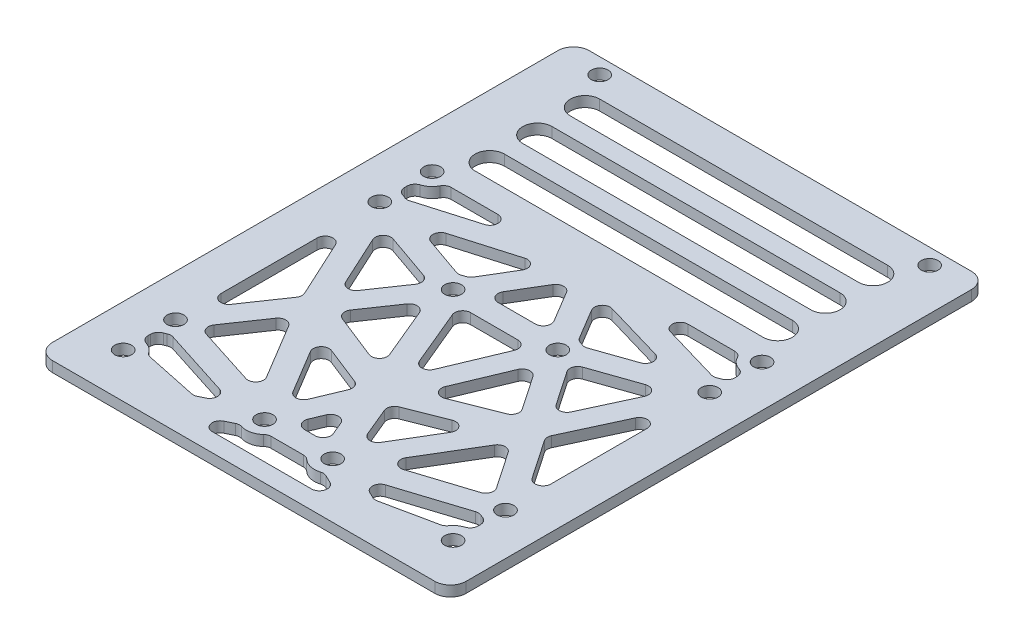
SolidWorks part; units mm, degrees
material "Thornel Mat VMA"
ref_plane "Front Plane" through (0, 0, 0) normal (0, 0, 1) x (1, 0, 0)
ref_plane "Top Plane" through (0, 0, 0) normal (0, 1, 0) x (1, 0, 0)
ref_plane "Right Plane" through (0, 0, 0) normal (1, 0, 0) x (0, 0, -1)
sketch "Sketch1" plane through (0, 0, 0) normal (0, 1, 0) x (1, 0, 0)
  line L0 (0, 56) -> (0, -46.5) construction
  line L1 (-39.5, 56) -> (39.5, 56)
  line L2 (-39.5, 56) -> (-39.5, -46.5)
  line L3 (-39.5, -46.5) -> (39.5, -46.5)
  line L4 (39.5, 56) -> (39.5, -46.5)
  line L5 (-31.5, 21) -> (-31.5, 11) construction
  line L6 (31.5, 21) -> (31.5, 11) construction
  line L7 (-10, 3.5) -> (10, 3.5) construction
  line L8 (-6.5, -36) -> (6.5, -36) construction
  line L9 (-31.5, -28) -> (-31.5, -38) construction
  line L10 (31.5, -28) -> (31.5, -38) construction
  circle A0 centre (-31.5, 11) radius 1.6
  circle A1 centre (-31.5, 21) radius 1.6
  circle A2 centre (31.5, 11) radius 1.6
  circle A3 centre (31.5, 21) radius 1.6
  circle A4 centre (-6.5, -36) radius 1.6
  circle A5 centre (6.5, -36) radius 1.6
  circle A6 centre (-10, 3.5) radius 1.6
  circle A7 centre (10, 3.5) radius 1.6
  circle A8 centre (-31.5, 53) radius 1.6
  circle A9 centre (31.5, 53) radius 1.6
  circle A10 centre (-31.5, -28) radius 1.6
  circle A11 centre (-31.5, -38) radius 1.6
  circle A12 centre (31.5, -38) radius 1.6
  circle A13 centre (31.5, -28) radius 1.6
  dimension "D2" = 8
  dimension "D3" = 3.2
  dimension "D5" = 20
  dimension "D12" = 3
  dimension "D13" = 2
  dimension "D1" = 79
  dimension "D4" = 10
  dimension "D6" = 3.5
  dimension "D7" = 52.5
  dimension "D8" = 46.5
  dimension "D9" = 13
  dimension "D10" = 10.5
  dimension "D11" = 11
  dimension "D14" = 28
extrude "Boss-Extrude1" add sketch "Sketch1" along normal blind 2
sketch "Sketch2" plane through (0, 2, 0) normal (0, 1, 0) x (1, 0, 0)
  line L0 (0, 56) -> (0, -46.5) construction
  line L1 (39.5, 56) -> (-39.5, 56) construction
  line L2 (-39.5, -46.5) -> (39.5, -46.5) construction
  line L3 (-27.5, 46.2) -> (27.5, 46.2) construction
  line L4 (-27.5, 49) -> (27.5, 49)
  line L5 (-27.5, 43.4) -> (27.5, 43.4)
  line L6 (-39.5, 56) -> (-39.5, -46.5) construction
  line L7 (-27.5, 37.1) -> (27.5, 37.1) construction
  line L8 (-27.5, 39.9) -> (27.5, 39.9)
  line L9 (-27.5, 34.3) -> (27.5, 34.3)
  line L10 (-27.5, 28) -> (27.5, 28) construction
  line L11 (-27.5, 30.8) -> (27.5, 30.8)
  line L12 (-27.5, 25.2) -> (27.5, 25.2)
  line L13 (-31.5, -38) -> (-16.9387, -41.0657) construction
  line L16 (-16, -43) -> (16, -43)
  line L19 (-31.0571, -35.8961) -> (-16.4957, -38.9619)
  line L22 (-31.9429, -40.1039) -> (-17.3816, -43.1696)
  line L25 (-31.5, 11) -> (-10, 3.5) construction
  line L28 (-30.7918, 13.03) -> (-9.2918, 5.53)
  line L31 (-10, 3.5) -> (10, 3.5) construction
  line L32 (-10, 5.65) -> (10, 5.65)
  line L33 (-10, 1.35) -> (10, 1.35)
  line L37 (-32.2082, 8.97) -> (-10.7082, 1.47)
  line L43 (-16.9387, -41.0657) -> (-6.5, -36) construction
  line L44 (-17.8773, -39.1315) -> (-7.4387, -34.0657)
  line L45 (-16, -43) -> (-5.5613, -37.9343)
  line L46 (16.9387, -41.0657) -> (6.5, -36) construction
  line L49 (-31.5, -28) -> (-10, 3.5) construction
  line L56 (-33.2758, -26.788) -> (-11.7758, 4.712)
  line L59 (-29.7242, -29.212) -> (-8.2242, 2.288)
  line L62 (-31.5, 11) -> (-31.5, -28)
  line L65 (-31.5, -28) -> (-6.5, -36) construction
  line L68 (-6.5, -36) -> (6.5, -36) construction
  line L69 (-6.5, -33.85) -> (6.5, -33.85)
  line L70 (-6.5, -38.15) -> (6.5, -38.15)
  line L71 (-30.8447, -25.9523) -> (-5.8447, -33.9523)
  line L72 (-32.1553, -30.0477) -> (-7.1553, -38.0477)
  line L73 (-31.5, -28) -> (-31.5, -38)
  line L74 (17.8773, -39.1315) -> (7.4387, -34.0657)
  line L75 (16, -43) -> (5.5613, -37.9343)
  line L76 (-10, 3.5) -> (6.5, -36) construction
  line L77 (-8.0161, 4.3287) -> (8.4839, -35.1713)
  line L78 (-11.9839, 2.6713) -> (4.5161, -36.8287)
  line L79 (-6.5, -36) -> (10, 3.5) construction
  line L80 (-8.4839, -35.1713) -> (8.0161, 4.3287)
  line L81 (-4.5161, -36.8287) -> (11.9839, 2.6713)
  line L82 (-31.5, 11) -> (-20.75, -12.25) construction
  line L83 (-29.5485, 11.9023) -> (-18.7985, -11.3477)
  line L84 (-33.4515, 10.0977) -> (-22.7015, -13.1523)
  line L85 (-20.75, -12.25) -> (-6.5, -36) construction
  line L86 (-18.9064, -11.1438) -> (-4.6564, -34.8938)
  line L87 (-22.5936, -13.3562) -> (-8.3436, -37.1062)
  line L88 (-20.75, -12.25) -> (0, -20.4394) construction
  line L89 (-19.9607, -10.2501) -> (0.7893, -18.4395)
  line L90 (-21.5393, -14.2499) -> (-0.7893, -22.4393)
  line L91 (-28.0927, 20.2) -> (28.0927, 20.2)
  line L92 (-31.5, 17.5) -> (-31.5, 14.5)
  line L93 (31.5, 17.5) -> (31.5, 14.5)
  line L94 (-31.5, 11) -> (0, 20.2) construction
  line L95 (-32.1028, 13.0638) -> (-0.6028, 22.2638)
  line L96 (-30.8972, 8.9362) -> (0.6028, 18.1362)
  line L97 (-10, 3.5) -> (0, 20.2) construction
  line L98 (-11.8446, 4.6045) -> (-1.8446, 21.3045)
  line L99 (-8.1554, 2.3955) -> (1.8446, 19.0955)
  line L100 (31.5, -28) -> (31.5, -38)
  line L101 (31.5, 11) -> (31.5, -28)
  line L102 (31.5, -38) -> (16.9387, -41.0657) construction
  line L103 (31.0571, -35.8961) -> (16.4957, -38.9619)
  line L104 (31.9429, -40.1039) -> (17.3816, -43.1696)
  line L105 (31.5, -28) -> (6.5, -36) construction
  line L106 (30.8447, -25.9523) -> (5.8447, -33.9523)
  line L107 (32.1553, -30.0477) -> (7.1553, -38.0477)
  line L108 (20.75, -12.25) -> (0, -20.4394) construction
  line L109 (19.9607, -10.2501) -> (-0.7893, -18.4395)
  line L110 (21.5393, -14.2499) -> (0.7893, -22.4393)
  line L111 (20.75, -12.25) -> (6.5, -36) construction
  line L112 (18.9064, -11.1438) -> (4.6564, -34.8938)
  line L113 (22.5936, -13.3562) -> (8.3436, -37.1062)
  line L114 (31.5, -28) -> (10, 3.5) construction
  line L115 (33.2758, -26.788) -> (11.7758, 4.712)
  line L116 (29.7242, -29.212) -> (8.2242, 2.288)
  line L117 (31.5, 11) -> (20.75, -12.25) construction
  line L118 (29.5485, 11.9023) -> (18.7985, -11.3477)
  line L119 (33.4515, 10.0977) -> (22.7015, -13.1523)
  line L120 (31.5, 11) -> (10, 3.5) construction
  line L121 (30.7918, 13.03) -> (9.2918, 5.53)
  line L122 (32.2082, 8.97) -> (10.7082, 1.47)
  line L123 (10, 3.5) -> (0, 20.2) construction
  line L124 (11.8446, 4.6045) -> (1.8446, 21.3045)
  line L125 (8.1554, 2.3955) -> (-1.8446, 19.0955)
  line L126 (31.5, 11) -> (0, 20.2) construction
  line L127 (32.1028, 13.0638) -> (0.6028, 22.2638)
  line L128 (30.8972, 8.9362) -> (-0.6028, 18.1362)
  arc A0 (-27.5, 49) -> (-27.5, 43.4) centre (-27.5, 46.2) ccw
  arc A1 (27.5, 43.4) -> (27.5, 49) centre (27.5, 46.2) ccw
  arc A2 (-27.5, 39.9) -> (-27.5, 34.3) centre (-27.5, 37.1) ccw
  arc A3 (27.5, 34.3) -> (27.5, 39.9) centre (27.5, 37.1) ccw
  arc A4 (-27.5, 30.8) -> (-27.5, 25.2) centre (-27.5, 28) ccw
  arc A5 (27.5, 25.2) -> (27.5, 30.8) centre (27.5, 28) ccw
  arc A18 (-10, 5.65) -> (-10, 1.35) centre (-10, 3.5) ccw
  arc A19 (10, 1.35) -> (10, 5.65) centre (10, 3.5) ccw
  arc A26 (-17.8773, -39.1315) -> (-16, -43) centre (-16.9387, -41.0657) ccw
  arc A27 (-5.5613, -37.9343) -> (-7.4387, -34.0657) centre (-6.5, -36) ccw
  circle A44 centre (-10, 3.5) radius 3.5
  circle A45 centre (-31.5, 11) radius 3.5
  circle A46 centre (-6.5, -36) radius 3.5
  circle A48 centre (10, 3.5) radius 3.5
  circle A49 centre (31.5, 11) radius 3.5
  circle A50 centre (6.5, -36) radius 3.5
  arc A54 (-6.5, -33.85) -> (-6.5, -38.15) centre (-6.5, -36) ccw
  arc A55 (6.5, -38.15) -> (6.5, -33.85) centre (6.5, -36) ccw
  circle A56 centre (-31.5, -28) radius 3.5
  circle A57 centre (-31.5, -38) radius 3.5
  circle A58 centre (31.5, -28) radius 3.5
  circle A59 centre (31.5, -38) radius 3.5
  arc A60 (-31.0571, -35.8961) -> (-31.9429, -40.1039) centre (-31.5, -38) ccw
  arc A61 (-17.3816, -43.1696) -> (-16.4957, -38.9619) centre (-16.9387, -41.0657) ccw
  arc A62 (-30.7918, 13.03) -> (-32.2082, 8.97) centre (-31.5, 11) ccw
  arc A63 (-10.7082, 1.47) -> (-9.2918, 5.53) centre (-10, 3.5) ccw
  arc A64 (-33.2758, -26.788) -> (-29.7242, -29.212) centre (-31.5, -28) ccw
  arc A65 (-8.2242, 2.288) -> (-11.7758, 4.712) centre (-10, 3.5) ccw
  arc A66 (-30.8447, -25.9523) -> (-32.1553, -30.0477) centre (-31.5, -28) ccw
  arc A67 (-7.1553, -38.0477) -> (-5.8447, -33.9523) centre (-6.5, -36) ccw
  arc A68 (17.8773, -39.1315) -> (16, -43) centre (16.9387, -41.0657) cw
  arc A69 (5.5613, -37.9343) -> (7.4387, -34.0657) centre (6.5, -36) cw
  arc A70 (-8.0161, 4.3287) -> (-11.9839, 2.6713) centre (-10, 3.5) ccw
  arc A71 (4.5161, -36.8287) -> (8.4839, -35.1713) centre (6.5, -36) ccw
  arc A72 (-8.4839, -35.1713) -> (-4.5161, -36.8287) centre (-6.5, -36) ccw
  arc A73 (11.9839, 2.6713) -> (8.0161, 4.3287) centre (10, 3.5) ccw
  arc A74 (-29.5485, 11.9023) -> (-33.4515, 10.0977) centre (-31.5, 11) ccw
  arc A75 (-22.7015, -13.1523) -> (-18.7985, -11.3477) centre (-20.75, -12.25) ccw
  arc A76 (-18.9064, -11.1438) -> (-22.5936, -13.3562) centre (-20.75, -12.25) ccw
  arc A77 (-8.3436, -37.1062) -> (-4.6564, -34.8938) centre (-6.5, -36) ccw
  arc A78 (-19.9607, -10.2501) -> (-21.5393, -14.2499) centre (-20.75, -12.25) ccw
  arc A79 (-0.7893, -22.4393) -> (0.7893, -18.4395) centre (0, -20.4394) ccw
  circle A80 centre (-31.5, 21) radius 3.5
  circle A81 centre (31.5, 21) radius 3.5
  arc A82 (-32.1028, 13.0638) -> (-30.8972, 8.9362) centre (-31.5, 11) ccw
  arc A83 (0.6028, 18.1362) -> (-0.6028, 22.2638) centre (0, 20.2) ccw
  arc A84 (-11.8446, 4.6045) -> (-8.1554, 2.3955) centre (-10, 3.5) ccw
  arc A85 (1.8446, 19.0955) -> (-1.8446, 21.3045) centre (0, 20.2) ccw
  arc A86 (31.0571, -35.8961) -> (31.9429, -40.1039) centre (31.5, -38) cw
  arc A87 (17.3816, -43.1696) -> (16.4957, -38.9619) centre (16.9387, -41.0657) cw
  arc A88 (30.8447, -25.9523) -> (32.1553, -30.0477) centre (31.5, -28) cw
  arc A89 (7.1553, -38.0477) -> (5.8447, -33.9523) centre (6.5, -36) cw
  arc A90 (19.9607, -10.2501) -> (21.5393, -14.2499) centre (20.75, -12.25) cw
  arc A91 (0.7893, -22.4393) -> (-0.7893, -18.4395) centre (0, -20.4394) cw
  arc A92 (18.9064, -11.1438) -> (22.5936, -13.3562) centre (20.75, -12.25) cw
  arc A93 (8.3436, -37.1062) -> (4.6564, -34.8938) centre (6.5, -36) cw
  arc A94 (33.2758, -26.788) -> (29.7242, -29.212) centre (31.5, -28) cw
  arc A95 (8.2242, 2.288) -> (11.7758, 4.712) centre (10, 3.5) cw
  arc A96 (29.5485, 11.9023) -> (33.4515, 10.0977) centre (31.5, 11) cw
  arc A97 (22.7015, -13.1523) -> (18.7985, -11.3477) centre (20.75, -12.25) cw
  arc A98 (30.7918, 13.03) -> (32.2082, 8.97) centre (31.5, 11) cw
  arc A99 (10.7082, 1.47) -> (9.2918, 5.53) centre (10, 3.5) cw
  arc A100 (11.8446, 4.6045) -> (8.1554, 2.3955) centre (10, 3.5) cw
  arc A101 (-1.8446, 19.0955) -> (1.8446, 21.3045) centre (0, 20.2) cw
  arc A102 (32.1028, 13.0638) -> (30.8972, 8.9362) centre (31.5, 11) cw
  arc A103 (-0.6028, 18.1362) -> (0.6028, 22.2638) centre (0, 20.2) cw
  point P8 (0, 46.2)
  point P18 (0, 37.1)
  point P25 (0, 28)
  point P37 (-24.2193, -39.5329)
  point P45 (0, -36)
  point P46 (-20.75, 7.25)
  point P51 (-20.75, -12.25)
  point P59 (-19, -32)
  point P68 (-1.75, -16.25)
  point P73 (11.7193, -38.5329)
  point P74 (0, 3.5)
  point P91 (1.75, -16.25)
  point P98 (-26.125, -0.625)
  point P105 (-11.7193, -38.5329)
  point P114 (-13.625, -24.125)
  point P119 (31.5, 11)
  point P120 (-10.375, -16.3447)
  point P144 (-31.5, 11)
  point P153 (-15.75, 15.6)
  point P158 (-5, 11.85)
  point P174 (24.2193, -39.5329)
  point P180 (19, -32)
  point P187 (10.375, -16.3447)
  point P194 (13.625, -24.125)
  point P201 (20.75, -12.25)
  point P207 (26.125, -0.625)
  point P214 (20.75, 7.25)
  point P221 (5, 11.85)
  point P228 (15.75, 15.6)
  dimension "D1" = 2.8
  dimension "D10" = 7
  dimension "D7" = 4.3
  dimension "D8" = 5
  dimension "D2" = 7
  dimension "D3" = 12
  dimension "D5" = 3.5
  dimension "D6" = 3.5
  dimension "D9" = 32
  dimension "D4" = 3
extrude "Cut-Extrude1" cut sketch "Sketch2" against normal through all contours L5 A1 L4 A0 | L9 A3 L8 A2 | L12 A5 L11 A4 | A80 L92 A45 L95 L91 | A81 L91 L127 A49 L93 | A44 L98 L96 L28 | L32 L125 L99 | L124 A48 L121 L128 | L37 L83 L56 | L59 L89 L78 | L77 L80 L33 | L84 L62 L56 | L118 L122 L115 | L109 L116 L81 | L101 L119 L115 | L87 L59 L71 | L90 L86 L80 | L81 L69 L78 | L112 L110 L77 | L106 L116 L113 | A57 L19 L44 L72 A56 L73 | L75 A50 L70 A46 L45 L16 | L103 A59 L100 A58 L107 L74
fillet "R1.5 cutout fillet" radius 1.5 75 edges at (-31.5, 1, 34.5) (-31.5, 1, 31.5) (-29.5249, 1, 30.8894) (-12.2709, 1, 36.4107) (-17.2155, 1, 38.8103) (-28.3545, 1, 36.4651) (0, 1, 26.0174) (3.2719, 1, 33.85) (-3.2719, 1, 33.85) (17.2155, 1, 38.8103) (12.2709, 1, 36.4107) (29.5249, 1, 30.8894) (31.5, 1, 31.5) (31.5, 1, 34.5) (28.3545, 1, 36.4651) (-16, 1, 43) (-8.046, 1, 39.14) (-3.7382, 1, 38.15) (3.7382, 1, 38.15) (8.046, 1, 39.14) (16, 1, 43) (0, 1, -16.015) (6.2066, 1, -5.65) (-6.2066, 1, -5.65) (4.6626, 1, -16.5984) (24.4523, 1, -10.8186) (11.8995, 1, -6.4397) (10.4257, 1, -6.974) (31.5, 1, -17.5) (31.5, 1, -14.5) (29.4517, 1, -13.8381) (7.669, 1, -20.2) (28.0927, 1, -20.2) (-11.2794, 1, 32.2132) (-28.099, 1, 26.8309) (-20.8666, 1, 16.2346) (31.5, 1, 24.1862) (23.2133, 1, 12.0453) (31.5, 1, -5.877) (-10.4572, 1, 0.9836) (-3.9461, 1, 16.5706) (-17.4565, 1, 11.2384) (20.3891, 1, 7.9075) (13.3578, 1, -2.3943) (27.4205, 1, -7.2999) (-23.2133, 1, 12.0453) (-31.5, 1, 24.1862) (-31.5, 1, -5.877) (6.7719, 1, -1.35) (0, 1, 14.8614) (-6.7719, 1, -1.35) (3.9461, 1, 16.5706) (10.4572, 1, 0.9836) (17.4565, 1, 11.2384) (-2.8291, 1, 21.6342) (-6.8446, 1, 31.2469) (-15.6476, 1, 16.5752) (-7.669, 1, -20.2) (-29.4517, 1, -13.8381) (-31.5, 1, -14.5) (-31.5, 1, -17.5) (-13.3578, 1, -2.3943) (-20.3891, 1, 7.9075) (-27.4205, 1, -7.2999) (-11.8995, 1, -6.4397) (-24.4523, 1, -10.8186) (-4.6626, 1, -16.5984) (-10.4257, 1, -6.974) (6.8446, 1, 31.2469) (2.8291, 1, 21.6342) (15.6476, 1, 16.5752) (11.2794, 1, 32.2132) (20.8666, 1, 16.2346) (28.099, 1, 26.8309) (-28.0927, 1, -20.2)
fillet "R3 outer edge fillet" radius 3 4 edges at (-39.5, 1, -56) (39.5, 1, -56) (39.5, 1, 46.5) (-39.5, 1, 46.5)
